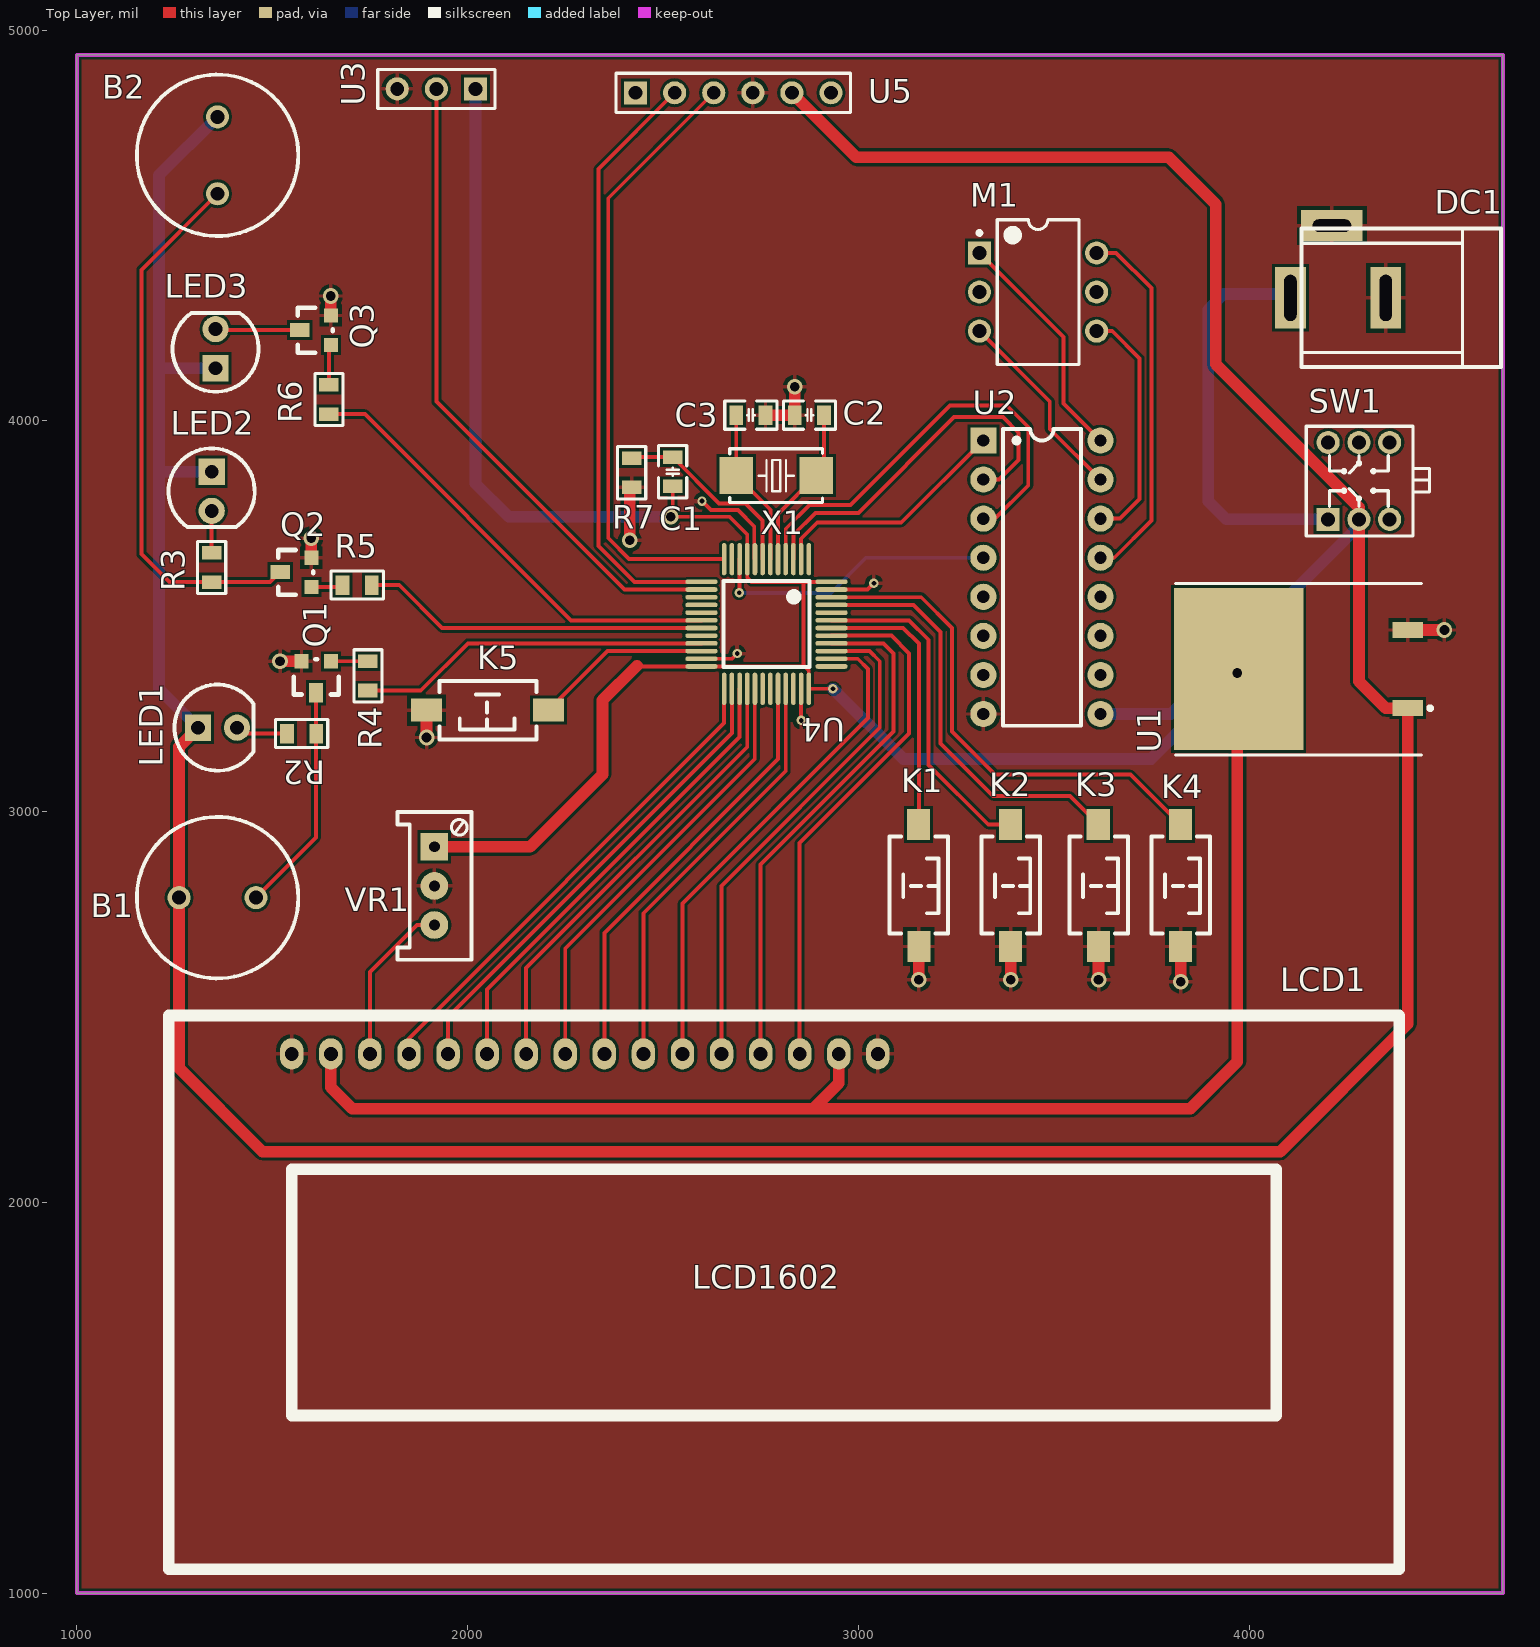
[diagram p0: Top Layer view]
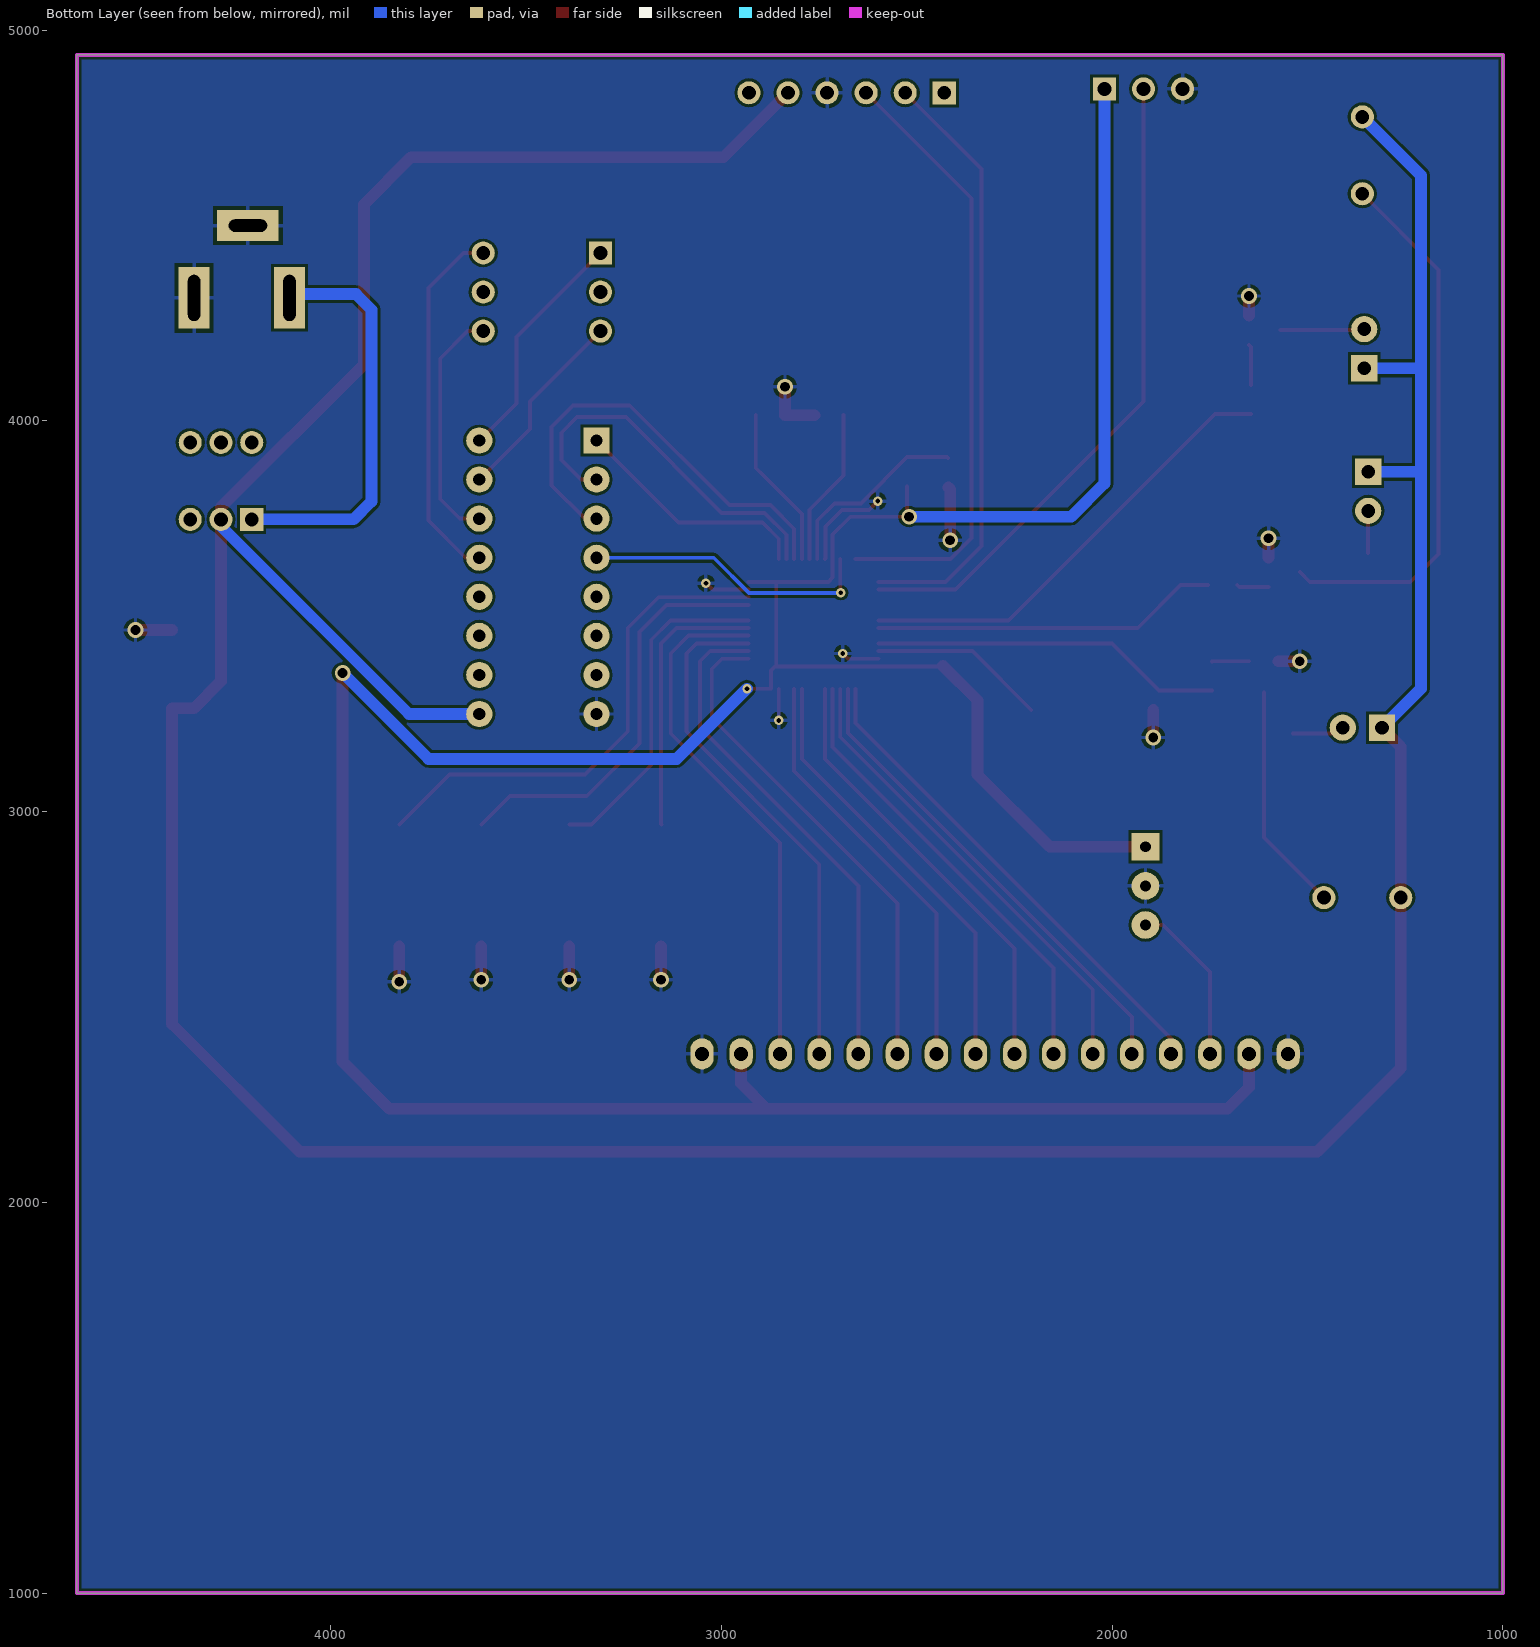
[diagram p1: Bottom Layer view, seen from below]
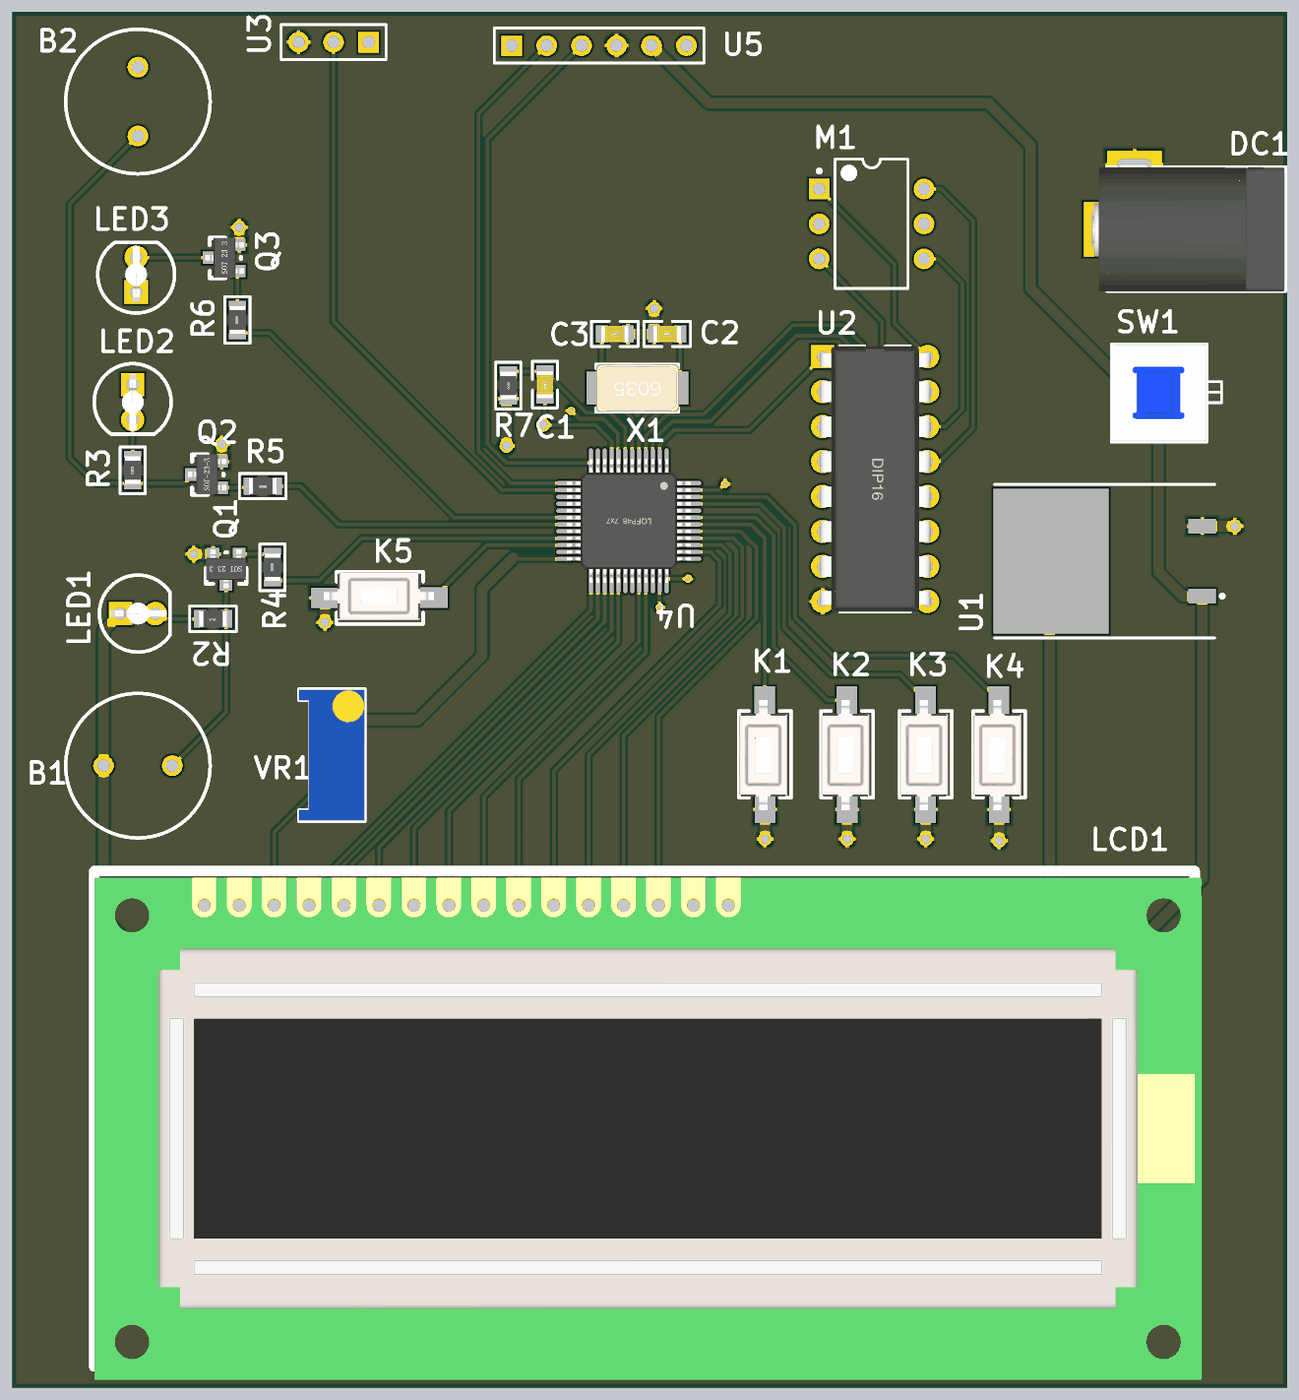
[diagram p2: 3D render of the assembled board from above, using the file's embedded part models]
# Altium PCB MISC80658.PcbDoc
Units mil, origin at the board's own origin, x right, y up, seen from the top; angles counter-clockwise.
Board outline 3650 x 3937.01 mil, 2 copper layers (Top Layer, Bottom Layer); 33 components, 53 nets, 159 pads, 19 vias.

## Layer stack, top to bottom (the 12.6 mil dielectric is the usual default, probably not edited)
Top Solder: solder mask 0.4, Solder Resist, Dk 3.5
Top Layer: signal copper 1.4
Dielectric 1: dielectric 12.6, FR-4, Dk 4.8
Bottom Layer: signal copper 1.4
Bottom Solder: solder mask 0.4, Solder Resist, Dk 3.5

## Board outline
1000,1000 1000,4937.01 4650,4937.01 4650,1000

## Design rules (kind name [scope] priority, off if disabled: settings)
Clearance [All] p1: gap=7
HoleSize [All] p1: absolutevalues=TRUE maxlimit=11111 minlimit=1 maxpercent=80.000 minpercent=20.000
MinimumSolderMaskSliver [All] p1: minsoldermaskwidth=0
PolygonConnect [All] p1: connectstyle=Relief reliefconductorwidth=10 reliefentries=4 polygonreliefangle="90 Angle" airgapwidth=10
RoutingVias [All] p1: holewidth=28 width=50 viastyle="Through Hole" minholewidth=28 minwidth=50 maxholewidth=28 maxwidth=50
SilkToSilkClearance [All] p1: silktosilkclearance=0
SilkToSolderMaskClearance [IsPad] p1: minsilkscreentomaskgap=0 clearancetoexposedcopper=TRUE
SolderMaskExpansion [All] p1: expansion=4
Width [All] p1: maxlimit=888 minlimit=10 preferedwidth=10
26 further rules are at their usual default settings.

## Components (designator, comment, footprint, x,y, rotation, side; value= is the part's Value field where it differs from the comment)
B1 "Fan" RB5-10.5 1360,2780 r0 top
B2 "Heater plate" RB5-10.5 1360,4680 r270 top
C1 "1uF" "C 0805_L" 2525,3870 r90 top
C2 "20pF" "C 0805_L" 2875,4015 r180 top
C3 "20pF" "C 0805_L" 2725,4015 r0 top
DC1 "DC005-2.5MM" DC-005 4105.91,4315 r0 top
K1 "SW-BUTTON" "TSW SMD-3*6*2.5" 3155,2810 r270 top
K2 "SW-BUTTON" "TSW SMD-3*6*2.5" 3390,2810 r270 top
K3 "SW-BUTTON" "TSW SMD-3*6*2.5" 3615,2810 r270 top
K4 "SW-BUTTON" "TSW SMD-3*6*2.5" 3825,2810 r270 top
K5 "SW-BUTTON" "TSW SMD-3*6*2.5" 2050,3260 r180 top
LCD1 "LCD1602" LCD1602 1550,2380 r0 top
LED1 "LED_G" "LED 5MM-W" 1360,3215 r0 top
LED2 "LED_G" "LED 5MM-W" 1345,3820 r270 top
LED3 "LED" "LED 5MM-W" 1355,4185 r90 top
M1 "STEP" DIP-6 3460,4330 r0 top
Q1 "8050" SOT-23 1615,3350 r180 top
Q2 "8050" SOT-23 1565,3610 r90 top
Q3 "8050" SOT-23 1615,4230 r90 top
R2 "510R" "R 0805_L" 1575,3200 r180 top
R3 "510R" "R 0805_L" 1345,3625 r90 top
R4 "10K" "R 0805_L" 1745,3347.4 r90 top
R5 "10K" "R 0805_L" 1717.4,3580 r180 top
R6 "10K" "R 0805_L" 1645,4055 r90 top
R7 "10K" "R 0805_L" 2420,3867.4 r270 top
SW1 "SW-DPDT" "KFT DIP-7X7" 4281.26,3846.57 r0 top
U1 "LM1117-3.3V" D2PAK 4190,3365 r90 top
U2 "ULN2003" DIP16 3470,3600 r0 top
U3 "DHT11" HDR1X3 2020,4850 r180 top
U4 "STM32F103C" "LQFP48 7X7" 2765,3480 r180 top
U5 "HC05 Bluetooth module" HDR1X6 2430,4840 r0 top
VR1 "50K" 3296W 1915,2810 r270 top
X1 "8MHz" "OSC 6035-2P" 2790,3860 r180 top

## Footprints (in the part's own frame and the unit in brackets; to place one, negate y for a bottom-side part, rotate by r counter-clockwise, add the part's x,y. Pads: shape width x height; smd on the part's side, far side on the other; paste and mask are expansions set on the pad)
3296W [mm] "Precise Multi-Winding Adjustable Resistor"
  rect 1.8x1.8 hole 0.7: 1(-2.54,0)
  round 1.8 hole 0.7: 2(0,0) 3(2.54,0)
  silkscreen extent -4.8,-2.4 4.8,2.4, body extent -4.75,-2.4 4.75,2.4, height 11.52
"C 0805_L" [mil] "无极性贴片电容"
  rect 35x50 smd: 1(-37.4,0) 2(37.4,0)
  silkscreen extent -67,-36 67,36, body extent -39,-24 39,24, height 20
D2PAK [mm] "D2-PAK/TO-263-AB; 3 Leads (1 Cropped); Body 15.5 (inc. leads) x 10.5 mm (LxW max)"
  rect 1.05x2 smd: 1(-2.54,-5.5) 3(2.54,-5.5)
  rect 10.55x8.4 smd: 2(0,5.5)
  silkscreen extent -5.58,-7.08 5.58,9.6
DC-005 [mm] "5.5X2.1mm"
  rect 2x4 hole 0.8 slot 3 at 90 deg: 1(0,0) 2(6.2,0)
  rect 4x2 hole 0.8 slot 2.5 at 0 deg: 3(2.7,4.7)
  silkscreen extent 0.72,-4.5 13.7,4.5, body extent -0.4,-4.52 13.65,4.78, height 11.2
DIP16 [mm]
  rect 1.7x1.7 hole 0.8: 1(-3.81,8.89)
  round 1.7 hole 0.8: 2(-3.81,6.35) 3(-3.81,3.81) 4(-3.81,1.27) 5(-3.81,-1.27) 6(-3.81,-3.81) 7(-3.81,-6.35) 8(-3.81,-8.89) 9(3.81,-8.89) 10(3.81,-6.35) 11(3.81,-3.81) 12(3.81,-1.27) 13(3.81,1.27) 14(3.81,3.81) 15(3.81,6.35) 16(3.81,8.89)
  silkscreen extent -2.54,-9.65 2.54,9.65, body extent -4.02,-9.65 4.02,9.65, height 4.45
DIP-6 [mm] "DIP; 6 Leads; Row Spacing 7.62 mm; Pitch 2.54 mm"
  rect 1.5x1.5 hole 0.9: 1(-3.81,2.54)
  round 1.5 hole 0.9: 2(-3.81,0) 3(-3.81,-2.54) 4(3.81,-2.54) 5(3.81,0) 6(3.81,2.54)
  silkscreen extent -3.93,-4.7 2.65,4.7, body extent -3.55,-4.7 3.55,4.7, height 5.46
HDR1X3 [mm] "Connector; Header; 3 Position"
  rect 1.5x1.5 hole 0.9: 1(0,0)
  round 1.5 hole 0.9: 2(2.54,0) 3(5.08,0)
  silkscreen extent -1.27,-1.27 6.35,1.27
HDR1X6 [mm] "Connector; Header; 6 Position"
  rect 1.5x1.5 hole 0.9: 1(0,0)
  round 1.5 hole 0.9: 2(2.54,0) 3(5.08,0) 4(7.62,0) 5(10.16,0) 6(12.7,0)
  silkscreen extent -1.27,-1.27 13.97,1.27
"KFT DIP-7X7" [mm] "自锁开关，规格：7*7mm"
  rect 1.5x1.5 hole 0.9: 1(-2,-2.5)
  round 1.5 hole 0.9: 2(0,-2.5) 3(2,-2.5) 4(2,2.5) 5(0,2.5) 6(-2,2.5)
  silkscreen extent -3.42,-3.58 4.58,3.56, body extent -3.5,-3.5 3.5,3.5, height 11.2
LCD1602 [mil]
  oval 60x80 hole 35.43: 1(0,0) 2(100,0) 3(200,0) 4(300,0) 5(400,0) 6(500,0) 7(600,0) 8(700,0) 9(800,0) 10(900,0) 11(1000,0) 12(1100,0) 13(1200,0) 14(1300,0) 15(1400,0) 16(1500,0)
  silkscreen extent -315,-1319 2835,98, body extent -315,-1357 2854,80, height 414
"LED 5MM-W" [mm] "白色5mm直插LED"
  rect 1.7x1.7 hole 0.9: 1(-1.27,0)
  round 1.7 hole 0.9: 2(1.27,0)
  silkscreen extent -2.8,-2.8 2.33,2.8, body extent -2.85,-2.85 2.45,2.85, height 8.75
"LQFP48 7X7" [mm]
  oval 0.3x2.1 smd: 1(-2.75,-4.227) 2(-2.25,-4.227) 3(-1.75,-4.227) 4(-1.25,-4.227) 5(-0.75,-4.227) 6(-0.25,-4.227) 7(0.25,-4.227) 8(0.75,-4.227) 9(1.25,-4.227) 10(1.75,-4.227) 11(2.25,-4.227) 12(2.75,-4.227) 25(2.75,4.202) 26(2.25,4.202) 27(1.75,4.202) 28(1.25,4.202) 29(0.75,4.202) 30(0.25,4.202) 31(-0.25,4.202) 32(-0.75,4.202) 33(-1.25,4.202) 34(-1.75,4.202) 35(-2.25,4.202) 36(-2.75,4.202)
  oval 2.1x0.3 smd: 13(4.227,-2.75) 14(4.227,-2.25) 15(4.227,-1.75) 16(4.227,-1.25) 17(4.227,-0.75) 18(4.227,-0.25) 19(4.227,0.25) 20(4.227,0.75) 21(4.227,1.25) 22(4.227,1.75) 23(4.227,2.25) 24(4.227,2.75) 37(-4.227,2.75) 38(-4.227,2.25) 39(-4.227,1.75) 40(-4.227,1.25) 41(-4.227,0.75) 42(-4.227,0.25) 43(-4.227,-0.25) 44(-4.227,-0.75) 45(-4.227,-1.25) 46(-4.227,-1.75) 47(-4.227,-2.25) 48(-4.227,-2.75)
  silkscreen extent -2.79,-2.79 2.79,2.79, body extent -4.51,-4.5 4.5,4.5, height 1.45
"OSC 6035-2P" [mm] "6mm*3.5mm*1mm(长*宽*高)"
  rect 2.2x2.4 smd: 1(-2.6,0) 2(2.6,0)
  silkscreen extent -3,-1.75 3.02,1.75, body extent -3,-1.75 3,1.75, height 1.06
"R 0805_L" [mil] "1/8W贴片电阻"
  rect 35x50 smd: 1(-37.4,0) 2(37.4,0)
  silkscreen extent -67,-36 67,36, body extent -39,-25 39,25, height 20
RB5-10.5 [mm] "Capacitor (Radial); 2 Leads"
  round 1.5 hole 0.9: 1(-2.5,0) 2(2.5,0)
  silkscreen extent -5.25,-5.25 5.25,5.25
SOT-23 [mil]
  rect 36x36 smd: B(-35,-35) E(40,-35)
  rect 36x50 smd: C(3,45)
  silkscreen extent -55,-40 60,50, body extent -54,-48 60,62, height 47
"TSW SMD-3*6*2.5" [mm] "3*6*2.5mm"
  rect 2x1.5 smd: 1(-3.996,-0.02) 2(3.937,0)
  silkscreen extent -3.21,-1.9 3.09,1.9, body extent -4,-1.88 4,1.62, height 2.59

## Part data
B1: library part Motor, "5V fan"
B2: library part Motor
C1 C2 C3: library part CAP, "Chip capacitor"
K1 K2 K3 K4 K5: "Tact switch"
LCD1: "LCD module"
LED1 LED2: "Green LED"
M1: library part "MOTOR STEPPER-4_-2", "Stepper motor"
Q1 Q2 Q3: library part NPN, "NPN transistor"
R2 R3 R4 R5 R6: library part RES, "Resistor"
R7: library part RES1
SW1: "DPDT switch"
U1: library part LM78xx, "Voltage regulator circuit"
U2: "ULN2003 driver IC"
U3: library part DS18B20, "DHT11 temperature/humidity"
U4: library part STM32F103C8T6, "48-pin LQFP"
U5: library part HC-05-蓝牙模块, "HC-05 Bluetooth module"
VR1: library part RW, "Potentiometer"
X1: library part CRYSTAL, "Crystal oscillator"

## Via types
v1: diameter 40, hole 25, Top Layer to Bottom Layer, 13 vias
v2: diameter 24, hole 12, Top Layer to Bottom Layer, 6 vias

## Nets (pads, with @x,y where several pads share a name; then routed paths per layer and width w, separated by ;. In a path a pad name is that pad's centre, name@x,y a point inside that pad or via, vN(x,y) a via of type N, cw(c..) or ccw(c..) an arc to the next point about the centre after c; other vN are vias at no path point)
3V3: C1.1 LCD1.2 LCD1.15 U1.2 U3.1 U4.9 U4.24 U4.36 U4.48 VR1.1 | length 8612.7
  Top Layer w10: 2433.51,3373.51 2435.29,3371.73 U4.24 2863.27,3371.73 ; C1.1 2525,3760 v1(2520,3755) 2670,3755 2715.79,3709.21 U4.9 2715.79,3599.21 2726.73,3588.27 2860,3588.27 ; U4.48 2860,3588.27 ; v2@2944.58,3314.58 U4.36 2873.27,3361.73 2863.27,3371.73 ; 2860,3588.27 2860,3375 2863.27,3371.73
  Top Layer w30: LCD1.2 1650,2295 1705,2240 2885,2240 ; VR1.1 2160,2910 2345,3095 2345,3285 2433.51,3373.51 ; LCD1.15 2950,2305 2885,2240 ; v1(3970,3355) 3970,2360 3850,2240 2885,2240
  Bottom Layer w30: U3.1 2020,3840 2105,3755 v1(2520,3755) ; v2(2935,3315) 3115,3135 3750,3135 v1(3970,3355)
5V: B1.1 B2.1 LED1.1 LED2.1 LED3.1 SW1.2 U1.1 U2.9 U5.5 | length 10625
  Top Layer w30: LED1.1 1261.57,3166.57 B1.1 1261.57,2343.43 1475,2130 4080,2130 4406.54,2456.54 U1.1 4350,3265 4281.26,3333.74 SW1.2 4281.26,3778.74 3915,4145 3915,4555 3795,4675 2995,4675 U5.5
  Bottom Layer w30: LED1.1 1210,3315 1210,3865 ; LED2.1 1215,3870 1210,3865 ; LED3.1 1210,4135 ; B2.1 1210,4628.43 1210,4135 ; U2.9 3800,3250 4281.26,3731.26 SW1.2 ; 1210,3865 1210,4135
GND: C2.2 C3.2 DC1.2 DC1.3 K1.2 K2.2 K3.2 K4.2 K5.2 LCD1.1 LCD1.16 Q1.E Q2.E Q3.E R7.2 U1.3 U2.8 U3.3 U4.8 U4.23 U4.35 U4.47 U5.4 VR1.2 | length 1486.9
  Top Layer w10: U4.23 2676.42,3391.42 v2(2690,3405) ; v2(2600,3795) 2623,3772 2692.04,3772 2733.69,3730.35 2733.69,3648.2 U4.8 ; v2(2853.58,3233.58) U4.35 ; U4.47 3023.58,3568.58 v2(3040,3585)
  Top Layer w30: v1(1520,3385) Q1.E ; Q2.E v1(1600,3700) ; Q3.E v1(1650,4320) ; v1(1895,3190) K5.2 ; v1(2415,3695) 2415,3825 R7.2 ; C3.2 C2.2 v1(2837.6,4087.6) ; v1(3155,2570) K1.2 ; v1(3390,2570) K2.2 ; v1(3615,2570) K3.2 ; v1(3825,2565) K4.2 ; U1.3 v1(4500,3465)
NetB1_2: B1.2 Q1.C R2.1 | length 588.6
  Top Layer w10: B1.2 1612,2933.57 Q1.C
NetB2_2: B2.2 Q2.C R3.1 | length 1397.9
  Top Layer w10: B2.2 1165,4386.57 1165,3660 1237.4,3587.6 R3.1 1494.6,3587.6 Q2.C
NetC1_2: C1.2 R7.1 U4.7 | length 502
  Top Layer w10: R7.1 2422.6,3907.4 C1.2 2643.4,3789 2711,3789 2755.16,3744.84 U4.7
NetC2_1: C2.1 U4.5 X1.1 | length 417.4
  Top Layer w10: U4.5 2794.53,3762.17 X1.1 2912.4,3880.04 C2.1
NetC3_1: C3.1 U4.6 X1.2 | length 404.7
  Top Layer w10: C3.1 C3.1 X1.2 2774.84,3772.8 U4.6
NetDC1_1: DC1.1 SW1.1 | length 1047.3
  Bottom Layer w30: DC1.1 4095.91,4325 3935.91,4325 3895.91,4285 3895.91,3794.09 3941.85,3748.15 SW1.1
NetLCD1_3: LCD1.3 VR1.3 | length 424.7
  Top Layer w10: LCD1.3 1750,2590 1870,2710 VR1.3
NetLED1_2: LED1.2 R2.2 | length 133.8
  Top Layer w10: LED1.2 1425,3200 R2.2
NetLED2_2: LED2.2 R3.2 | length 107.6
  Top Layer w10: R3.2 LED2.2
NetLED3_2: LED3.2 Q3.C | length 215.8
  Top Layer w10: LED3.2 1357,4233 Q3.C
NetM1_1: M1.1 U2.16 | length 608.4
  Top Layer w10: M1.1 3525,4215 3525,4045 U2.16
NetM1_3: M1.3 U2.15 | length 508.4
  Top Layer w10: M1.3 3490,4050 3490,3980 U2.15
NetM1_4: M1.4 U2.14 | length 619.7
  Top Layer w10: M1.4 3650,4230 3720,4160 3720,3800 3670,3750 U2.14
NetM1_6: M1.6 U2.13 | length 941.6
  Top Layer w10: M1.6 3660,4430 3750,4340 3750,3745 3655,3650 U2.13
NetQ1_B: Q1.B R4.2 | length 95.1
  Top Layer w10: Q1.B 1744.8,3385 R4.2
NetQ2_B: Q2.B R5.2 | length 82.1
  Top Layer w10: Q2.B 1675,3575 R5.2
NetQ3_B: Q3.B R6.2 | length 104.7
  Top Layer w10: R6.2 1645,4190 Q3.B
PA0: U2.4 U4.10 | length 749.2
  Top Layer w10: v2(2695,3560) 2696.1,3561.1 U4.10
  Bottom Layer w10: v2(2695,3560) 2930,3560 3020,3650 U2.4
PA1: U4.11
PA2: U4.12 U5.3 | length 1570.8
  Top Layer w10: U5.3 2360,4570 2360,3700 2413.58,3646.42 U4.12
PA3: U4.13 U5.2 | length 1542.4
  Top Layer w10: U5.2 2335,4645 2335,3680 2426.73,3588.27 U4.13
PA4: U3.2 U4.14 | length 1678
  Top Layer w10: U3.2 1920,4050 2401.42,3568.58 U4.14
PA5: U4.15
PA6: U4.16
PA7: U4.17
PA8: LCD1.8 U4.29 | length 1135.7
  Top Layer w10: LCD1.8 2250,2650 2735,3135 2735,3314.11 U4.29
PA9: U4.30
PA10: U4.31
PA11: LCD1.9 U4.32 | length 1118.7
  Top Layer w10: LCD1.9 2350,2690 2794.53,3134.53 U4.32
PA12: LCD1.10 U4.33 | length 1085.4
  Top Layer w10: LCD1.10 2450,2740 2814.21,3104.21 U4.33
PA15: LCD1.11 U4.38 | length 1286.3
  Top Layer w10: LCD1.11 2550,2765 3025,3240 3025,3365 2998.58,3391.42 U4.38
PB0: R6.1 U4.18 | length 1172.2
  Top Layer w10: R6.1 1737.4,4017.6 2265.16,3489.84 U4.18
PB1: R5.1 U4.19 | length 889.3
  Top Layer w10: R5.1 1825,3580 1934.84,3470.16 U4.19
PB2: U4.20
PB3: LCD1.12 U4.39 | length 1307.2
  Top Layer w10: LCD1.12 2650,2810 3055,3215 3055,3385 3028.9,3411.1 U4.39
PB4: LCD1.13 U4.40 | length 1335.1
  Top Layer w10: LCD1.13 2750,2865 3090,3205 3090,3405 3064.21,3430.79 U4.40
PB5: LCD1.14 U4.41 | length 1358.4
  Top Layer w10: LCD1.14 2850,2920 3130,3200 3130,3405 3084.53,3450.47 U4.41
PB6: K1.1 U4.42 | length 703.2
  Top Layer w10: U4.42 3114.84,3470.16 3155,3430 3155,2968.1 K1.1
PB7: K2.1 U4.43 | length 861.7
  Top Layer w10: U4.43 3130.16,3489.84 3180,3440 3180,3120 3332.69,2967.31 K2.1
PB8: K3.1 U4.45 | length 1082.5
  Top Layer w10: U4.45 3140.79,3529.21 3210,3460 3210,3175 3345,3040 3541.53,3040 K3.1
PB9: K4.1 U4.46 | length 1288.9
  Top Layer w10: U4.46 3161.1,3548.9 3240,3470 3240,3205 3350,3095 3696.53,3095 K4.1
PB10: R4.1 U4.21 | length 903.6
  Top Layer w10: R4.1 1880,3310 2000.79,3430.79 U4.21
PB11: K5.1 U4.22 | length 453.5
  Top Layer w10: K5.1 2357.63,3411.1 U4.22
PB12: LCD1.4 U4.25 | length 1268.7
  Top Layer w10: LCD1.4 1850,2420 2656.73,3226.73 U4.25
PB13: LCD1.5 U4.26 | length 1235.5
  Top Layer w10: LCD1.5 1950,2475 2676.42,3201.42 U4.26
PB14: LCD1.6 U4.27 | length 1202.2
  Top Layer w10: LCD1.6 2050,2545 2696.1,3191.1 U4.27
PB15: LCD1.7 U4.28 | length 1168.9
  Top Layer w10: LCD1.7 2150,2600 2715.79,3165.79 U4.28
PC13: U2.1 U4.2 | length 622.7
  Top Layer w10: U4.2 2853.58,3698.58 2895,3740 3110,3740 U2.1
PC14: U2.2 U4.3 | length 960.6
  Top Layer w10: U4.3 2833.9,3708.9 2890,3765 3000,3765 3245,4010 3370,4010 3410,3970 3410,3900 3360,3850 U2.2
PC15: U2.3 U4.4 | length 1152.4
  Top Layer w10: U4.4 2814.21,3724.21 2875,3785 2980,3785 3235,4040 3380,4040 3435,3985 3435,3835 3350,3750 U2.3
pads on no net: M1.2 M1.5 SW1.3 SW1.4 SW1.5 SW1.6 U2.5 U2.6 U2.7 U2.10 U2.11 U2.12 U4.1 U4.34 U4.37 U4.44 U5.1 U5.6

## Polygon pours and split planes (outlines as drawn)
GND on Top Layer "D" (solid, remove dead copper, pour order 0): 770,5185 855,5270 4770,5270 4770,860 4915,715 4895,695 860,695
GND on Bottom Layer "D" (solid, remove dead copper, pour order 2): 790,5095 850,5155 4900,5155 4900,695 4945,650 4920,675 590,675

## Keep-outs
Keep-Out Layer:
  the board outline again, w10